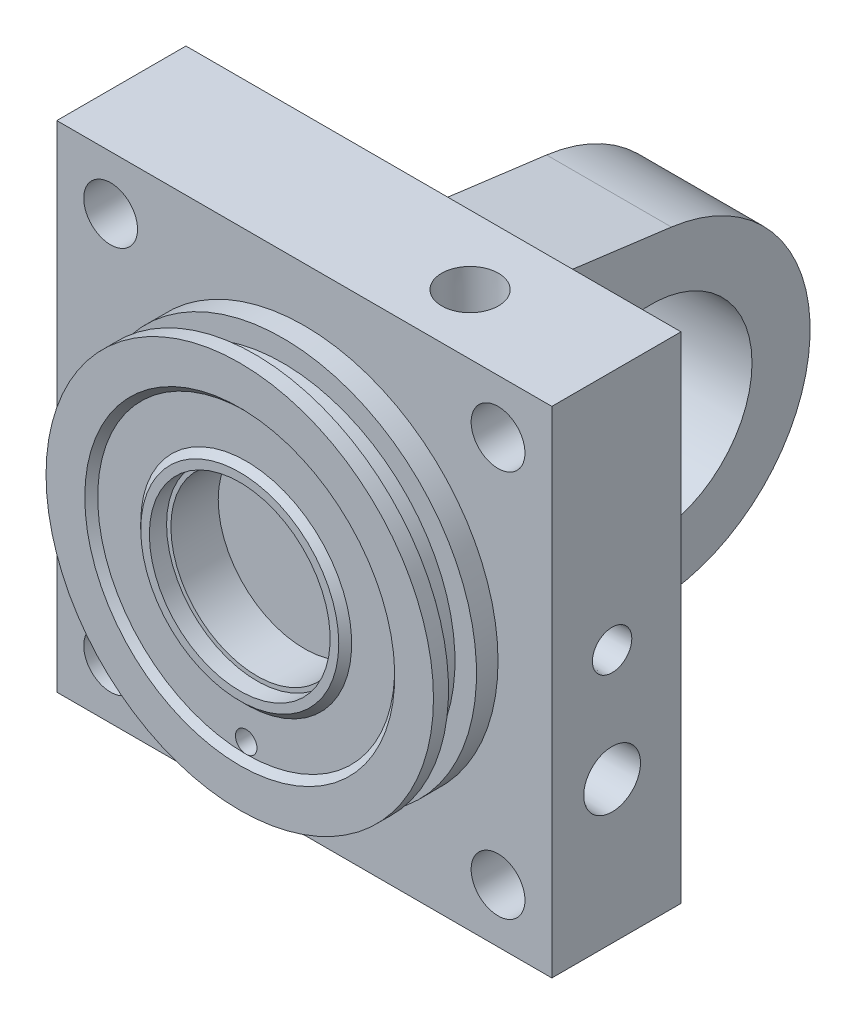
from build123d import *

# Parameters (mm, degrees)
SKETCH_1_W          = 115
SKETCH_1_H          = 115
SKETCH_1_R          = 6.25
EXTRUDE_1_DEPTH     = 30
SKETCH_2_R          = 45
EXTRUDE_2_DEPTH     = 15
SKETCH_3_W          = 6.5
SKETCH_3_H          = 5
SKETCH_4_R          = 2.5
CUT_EXTRUDE_1_DEPTH = 25
SKETCH_17_R         = 3
CUT_EXTRUDE_2_DEPTH = 43
SKETCH_18_R         = 3
CUT_EXTRUDE_3_DEPTH = 69
SKETCH_19_R         = 3
CUT_EXTRUDE_4_DEPTH = 82
SKETCH_20_R         = 23.5
EXTRUDE_3_DEPTH     = 14.5


with BuildPart() as part:
    # 草图1 → 凸台-拉伸1 (new body)
    with BuildSketch(Plane.XY):
        Rectangle(SKETCH_1_W, SKETCH_1_H)
        with Locations((-45, 45)):
            Circle(SKETCH_1_R, mode=Mode.SUBTRACT)
        with Locations((45, 45)):
            Circle(SKETCH_1_R, mode=Mode.SUBTRACT)
        with Locations((45, -45)):
            Circle(SKETCH_1_R, mode=Mode.SUBTRACT)
        with Locations((-45, -45)):
            Circle(SKETCH_1_R, mode=Mode.SUBTRACT)
    extrude(amount=EXTRUDE_1_DEPTH)

    # 草图2 → 凸台-拉伸2 (add)
    with BuildSketch(Plane.XY.offset(30)):
        Circle(SKETCH_2_R)
    extrude(amount=EXTRUDE_2_DEPTH)

    # 草图3 → 切除-旋转1 (revolve, cut)
    with BuildSketch(Plane(origin=(0, 0, 0), x_dir=(0, 0, -1), z_dir=(1, 0, 0)), mode=Mode.PRIVATE) as cut_revolve_1_sk:
        Polygon((-43.5, 34.5), (-45, 36), (-45, 23), (-43.5, 24.5), align=None)
        Polygon((-30, 0), (-45, 0), (-45, 21), (-41, 21), (-41, 20), (-30, 20), align=None)
        with Locations((-38.25, 42.5)):
            Rectangle(SKETCH_3_W, SKETCH_3_H)
    revolve(cut_revolve_1_sk.sketch.rotate(Axis((0, 0, 0), (0, 0, 1)), 90), axis=Axis((0, 0, 0), (0, 0, 1)), mode=Mode.SUBTRACT)

    # 草图4 → 切除-拉伸1 (cut)
    with BuildSketch(Plane.XY.offset(43.5)):
        with Locations((0, -32)):
            Circle(SKETCH_4_R)
    extrude(amount=-CUT_EXTRUDE_1_DEPTH, mode=Mode.SUBTRACT)

    # 草图6 → 1/4 NPT 螺纹孔1 (revolve, cut)
    with BuildSketch(Plane(origin=(-7.5, -57.5, 16), x_dir=(0, 0, -1), z_dir=(1, 0, 0))):
        Polygon((0, 0), (0, 35.390848279), (5.5626, 32.048501), (5.5626, 25), (5.943680721, 25), (6.6922142, 0), align=None)
    revolve(axis=Axis((-7.5, -63.85, 16), (0, 1, 0)), mode=Mode.SUBTRACT)

    # 草图9 → 1/4 Rc 螺纹孔1 (revolve, cut)
    with BuildSketch(Plane(origin=(57.5, -24.5, 16), x_dir=(0, 0, -1), z_dir=(0, 1, 0))):
        Polygon((0, 0), (0, 34.899604312), (5.35, 31.685), (5.35, 25), (5.810616973, 25), (6.5910325, 0), align=None)
    revolve(axis=Axis((63.85, -24.5, 16), (-1, 0, 0)), mode=Mode.SUBTRACT)

    # 草图12 → 1/8 Rc 螺纹孔1 (revolve, cut)
    with BuildSketch(Plane(origin=(57.5, 1.5, 16), x_dir=(0, 0, -1), z_dir=(0, 1, 0))):
        Polygon((0, 0), (0, 14.313399445), (3.95, 11.94), (3.95, 7.4), (4.342497004, 7.4), (4.5735, 0), align=None)
    revolve(axis=Axis((63.85, 1.5, 16), (-1, 0, 0)), mode=Mode.SUBTRACT)

    # 草图15 → 1/4 Rc 螺纹孔2 (revolve, cut)
    with BuildSketch(Plane(origin=(24.5, 57.5, 16), x_dir=(0, 0, 1), z_dir=(1, 0, 0))):
        Polygon((0, 0), (0, 34.899604312), (5.35, 31.685), (5.35, 25), (5.810616973, 25), (6.5910325, 0), align=None)
    revolve(axis=Axis((24.5, 63.85, 16), (0, -1, 0)), mode=Mode.SUBTRACT)

    # 草图17 → 切除-拉伸2 (cut)
    with BuildSketch(Plane(origin=(0, 57.5, 0), x_dir=(1, 0, 0), z_dir=(0, 1, 0))):
        with Locations(Location((24.5, -16, 0), (0, 0, 270))):
            Circle(SKETCH_17_R)
    extrude(amount=-CUT_EXTRUDE_2_DEPTH, mode=Mode.SUBTRACT)

    # 草图18 → 切除-拉伸3 (cut)
    with BuildSketch(Plane(origin=(57.5, 0, 0), x_dir=(0, 0, -1), z_dir=(1, 0, 0))):
        with Locations((-16, 1.5)):
            Circle(SKETCH_18_R)
        with Locations((-16, -24.5)):
            Circle(SKETCH_18_R)
    extrude(amount=-CUT_EXTRUDE_3_DEPTH, mode=Mode.SUBTRACT)

    # 草图19 → 切除-拉伸4 (cut)
    with BuildSketch(Plane.XZ.offset(57.5)):
        with Locations(Location((-7.5, 16, 0), (0, 0, 270))):
            Circle(SKETCH_19_R)
    extrude(amount=-CUT_EXTRUDE_4_DEPTH, mode=Mode.SUBTRACT)

    # 草图20 → 凸台-拉伸3 (add, symmetric)
    with BuildSketch(Plane(origin=(0, 0, 0), x_dir=(0, 0, -1), z_dir=(1, 0, 0))):
        with BuildLine():
            Line((0, 42), (0, -42))
            Line((0, -42), (40.777526531, -36.690260836))
            ThreePointArc((40.777526531, -36.690260836), (73, 0), (40.777526531, 36.690260836))
            Line((40.777526531, 36.690260836), (0, 42))
        make_face()
        with Locations(Location((36, 0, 0), (0, 0, 180))):
            Circle(SKETCH_20_R, mode=Mode.SUBTRACT)
    extrude(amount=EXTRUDE_3_DEPTH, both=True)


solid = part.part
